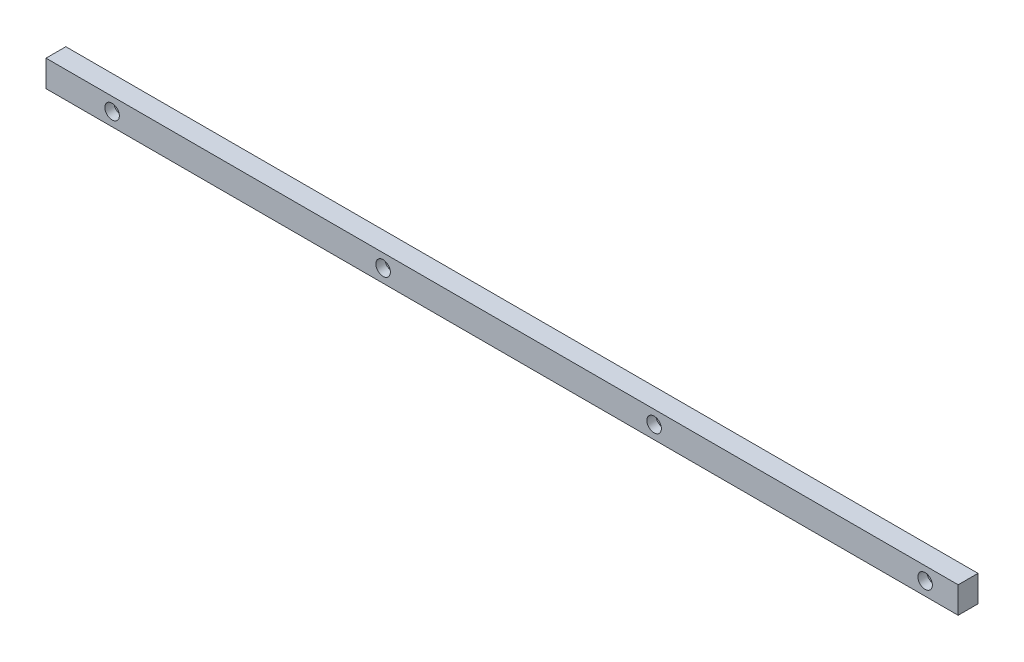
from build123d import *

# Parameters (mm, degrees)
SKETCH_1_W                = 665
SKETCH_1_H                = 20
EXTRUDE_1_DEPTH           = 15
HOLE_WIZARD_1_D           = 6.6
HOLE_WIZARD_1_CBORE_D     = 11
HOLE_WIZARD_1_CBORE_DEPTH = 6.8
SKETCH_5_W                = 15
SKETCH_5_H                = 20
EXTRUDE_2_DEPTH           = 25


with BuildPart() as part:
    # 草图1 → 凸台-拉伸1 (new body)
    with BuildSketch(Plane.XY):
        Rectangle(SKETCH_1_W, SKETCH_1_H)
    extrude(amount=EXTRUDE_1_DEPTH)

    # 打孔尺寸(%根据)内六角圆柱头螺钉的类型1 (through all)
    with Locations(Plane.XY.offset(15)):
        with Locations((102.5, 0), (-307.5, 0), (307.5, 0), (-102.5, 0)):
            CounterBoreHole(HOLE_WIZARD_1_D / 2, HOLE_WIZARD_1_CBORE_D / 2, HOLE_WIZARD_1_CBORE_DEPTH)

    # 草图5 → 凸台-拉伸2 (add)
    with BuildSketch(Plane.ZY.offset(332.5)):
        with Locations((7.5, 0)):
            Rectangle(SKETCH_5_W, SKETCH_5_H)
    extrude(amount=EXTRUDE_2_DEPTH)


solid = part.part
